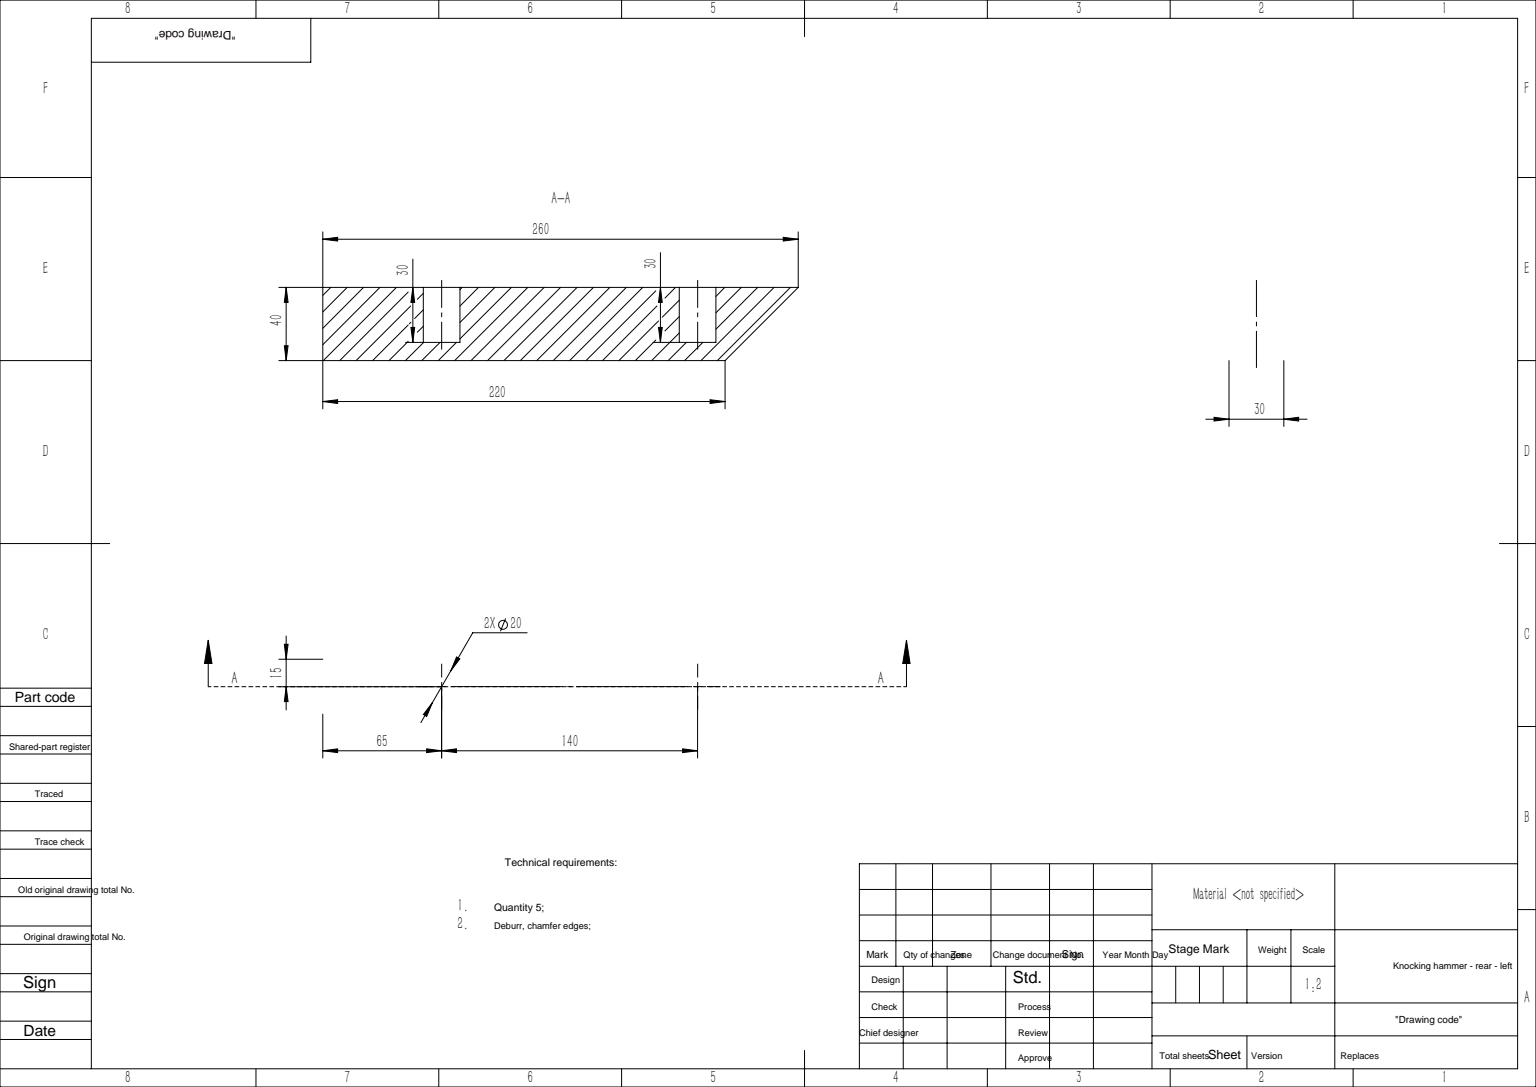
SolidWorks part; units mm, degrees
ref_plane "前视基准面" through (0, 0, 0) normal (0, 0, 1) x (1, 0, 0)
ref_plane "上视基准面" through (0, 0, 0) normal (0, 1, 0) x (1, 0, 0)
ref_plane "右视基准面" through (0, 0, 0) normal (1, 0, 0) x (0, 0, -1)
sketch "草图1" plane through (0, 0, 0) normal (0, 1, 0) x (1, 0, 0)
  line L1 (-135, -15) -> (135, -15)
  line L2 (-135, -15) -> (-135, 15)
  line L3 (-135, 15) -> (135, 15)
  line L4 (135, -15) -> (135, 15)
  line L5 (-135, -15) -> (135, 15) construction
  line L6 (-135, 15) -> (135, -15) construction
  point P0 (0, 0)
  dimension "D1" = 270
  dimension "D2" = 30
extrude "凸台-拉伸1" add sketch "草图1" along normal blind 40
sketch "草图2" plane through (0, 40, 0) normal (0, 1, 0) x (1, 0, 0)
  line L1 (0, 0) -> (0, 40) construction
  circle A0 centre (70, 0) radius 10
  circle A1 centre (-70, 0) radius 10
  dimension "D1" = 20
  dimension "D2" = 140
  dimension "D3" = 40
extrude "切除-拉伸2" cut sketch "草图2" against normal blind 30
sketch "草图5" plane through (135, 0, 0) normal (1, 0, 0) x (0, 0, -1)
  line L4 (-15, 0) -> (15, 0)
  line L5 (15, 0) -> (15, 40)
  line L6 (15, 40) -> (-15, 40)
  line L7 (-15, 40) -> (-15, 0)
  line L8 (-15, 0) -> (15, 0)
  line L9 (15, 0) -> (15, 40)
  line L10 (15, 40) -> (-15, 40)
  line L11 (-15, 40) -> (-15, 0)
  dimension "D1" = 0
extrude "切除-拉伸4" cut sketch "草图5" against normal blind 10
sketch "草图6" plane through (0, 0, 15) normal (0, 0, 1) x (1, 0, 0)
  line L0 (125, 40) -> (85, 0)
  line L1 (-135, 0) -> (125, 0) construction
  line L2 (85, 0) -> (125, 0)
  line L3 (125, 0) -> (125, 40)
  dimension "D1" = 45
extrude "切除-拉伸5" cut sketch "草图6" against normal through all
